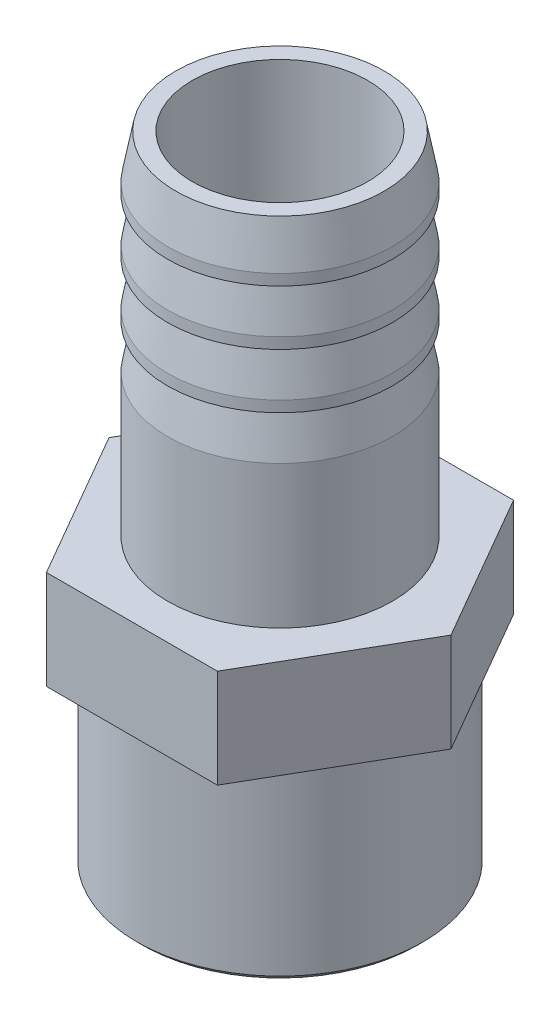
SolidWorks part; units mm, degrees
material "黄铜"
ref_plane "前视基准面" through (0, 0, 0) normal (0, 0, 1) x (1, 0, 0)
ref_plane "上视基准面" through (0, 0, 0) normal (0, 1, 0) x (1, 0, 0)
ref_plane "右视基准面" through (0, 0, 0) normal (1, 0, 0) x (0, 0, -1)
sketch "草图1" plane through (0, 0, 0) normal (0, 0, 1) x (1, 0, 0)
  line L0 (0, -266.5887) -> (0, 13062.8486) construction
  line L1 (-10.25, 13) -> (-9.5, 17)
  line L2 (0, 0) -> (-10.25, 0)
  line L3 (0, 0) -> (0, 32)
  line L5 (-10.25, 0) -> (-10.25, 13)
  line L6 (-10.25, 18) -> (-9.5, 22)
  line L7 (-10.25, 17) -> (-9.5, 17)
  line L8 (-10.25, 17) -> (-10.25, 18)
  line L11 (-9.5, -983) -> (-9.5, 49017) construction
  line L12 (-10.25, 22) -> (-9.5, 22)
  line L13 (-10.25, 22) -> (-10.25, 23)
  line L16 (-10.25, 23) -> (-9.5, 27)
  line L17 (-10.25, 27) -> (-9.5, 27)
  line L18 (-10.25, 27) -> (-10.25, 28)
  line L19 (-10.25, 28) -> (-9.5, 32)
  line L20 (-9.5, 32) -> (0, 32)
  dimension "D1" = 10.25
  dimension "D2" = 13
  dimension "D3" = 1
  dimension "D4" = 4
  dimension "D5" = 9.5
  dimension "D6" = 1
  dimension "D7" = 4
  dimension "D8" = 4
  dimension "D9" = 1
  dimension "D10" = 4
revolve "旋转1" add sketch "草图1" angle 360 about L3
sketch "草图2" plane through (0, 0, 0) normal (0, -1, 0) x (1, 0, 0)
  line L0 (-1000, 0) -> (49000, 0) construction
  line L1 (15.5885, 0) -> (7.7942, 13.5)
  line L2 (7.7942, 13.5) -> (-7.7942, 13.5)
  line L3 (-7.7942, 13.5) -> (-15.5885, 0)
  line L4 (-15.5885, 0) -> (-7.7942, -13.5)
  line L5 (-7.7942, -13.5) -> (7.7942, -13.5)
  line L6 (7.7942, -13.5) -> (15.5885, 0)
  circle A0 centre (0, 0) radius 13.5 construction
  dimension "D1" = 27
extrude "凸台-拉伸1" add sketch "草图2" along normal blind 9
sketch "草图3" plane through (0, -9, 0) normal (0, -1, 0) x (1, 0, 0)
  circle A0 centre (0, 0) radius 13.05
  dimension "D1" = 26.1
extrude "凸台-拉伸2" add sketch "草图3" along normal blind 17
cosmetic thread "装饰螺纹线1" parameters "D2"=24.117
sketch "草图4" plane through (0, 32, 0) normal (0, 1, 0) x (1, 0, 0)
  circle A0 centre (0, 0) radius 8
  dimension "D1" = 16
extrude "切除-拉伸1" cut sketch "草图4" against normal up to next
sketch "草图5" plane through (0, -26, 0) normal (0, -1, 0) x (1, 0, 0)
  circle A0 centre (0, 0) radius 9
  dimension "D1" = 18
extrude "切除-拉伸2" cut sketch "草图5" against normal up to surface (17 mm away) up to face at (13.05, -9, 0)
chamfer "倒角1" distance 0.5 angle 45 1 edges at (13.05, -26, 0)
chamfer "倒角2" distance 0.5 angle 45 1 edges at (8, -9, 0)
